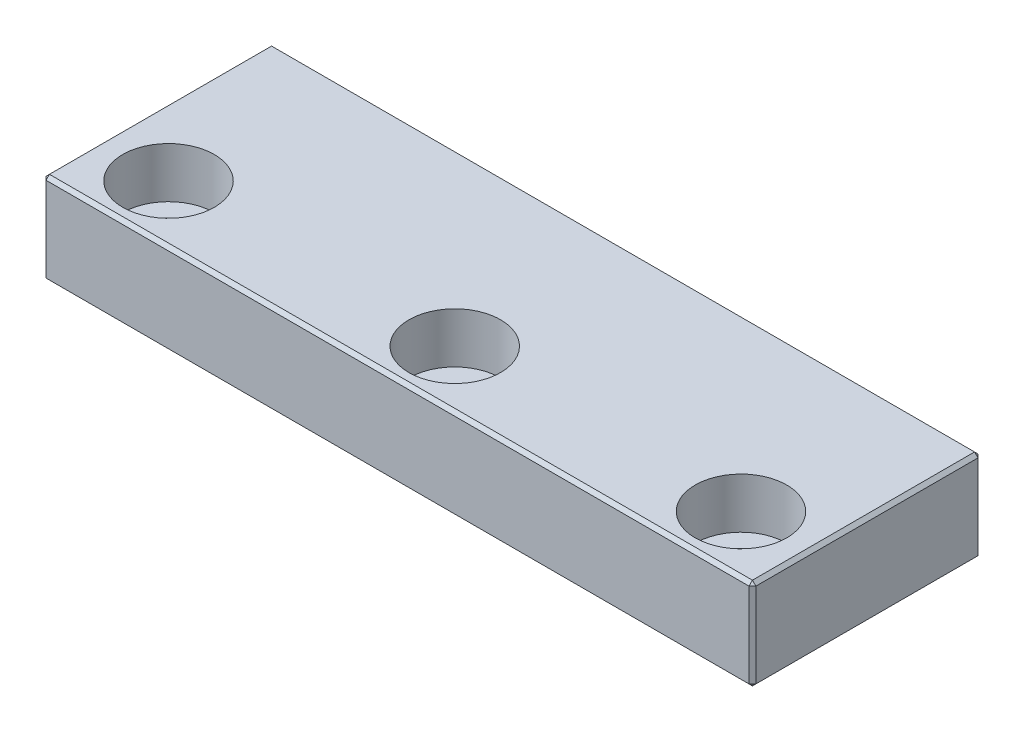
SolidWorks part; units mm, degrees
material "Al6061"
ref_plane "Front" through (0, 0, 0) normal (0, 0, 1) x (1, 0, 0)
ref_plane "Top" through (0, 0, 0) normal (0, 1, 0) x (1, 0, 0)
ref_plane "Right" through (0, 0, 0) normal (1, 0, 0) x (0, 0, -1)
sketch "草图1" plane through (0, 0, 0) normal (0, 1, 0) x (1, 0, 0)
  line L1 (-31, 10) -> (31, 10)
  line L2 (-31, 10) -> (-31, -10)
  line L3 (-31, -10) -> (31, -10)
  line L4 (31, 10) -> (31, -10)
  line L5 (-31, 10) -> (31, -10) construction
  line L6 (-31, -10) -> (31, 10) construction
  point P0 (0, 0)
  dimension "D1" = 62
  dimension "D2" = 20
extrude "凸台-拉伸1" add sketch "草图1" along normal blind 8
hole_wizard "M4 六角凹头螺钉的柱形沉头孔1" positions "草图3" profile "草图2" counterbore size "M4" standard "Iso" end condition through all
sketch "草图3" plane through (0, 8, 0) normal (0, 1, 0) x (1, 0, 0)
  line L0 (0, 0) -> (0, -5) construction
  line L2 (-31, -10) -> (31, -10) construction
  point P0 (-25, -5)
  point P2 (0, -5)
  point P4 (25, -5)
  dimension "D1" = 25
  dimension "D2" = 25
  dimension "D3" = 5
sketch "草图2" plane through (-25, 8, 5) normal (1, 0, 0) x (0, 0, 1)
  line L0 (0, 0) -> (0, 8)
  line L1 (0, 8) -> (2.25, 8)
  line L3 (2.25, 8) -> (2.25, 4.4)
  line L4 (2.25, 4.4) -> (4, 4.4)
  line L5 (4, 4.4) -> (4, 0)
  line L7 (4, 0) -> (0, 0)
  line L11 (0, -6.35) -> (0, 107.95) construction
  dimension "通孔孔直径" = 4.5
  dimension "通孔孔深度" = 8
  dimension "柱形沉头孔直径" = 8
  dimension "柱形沉头孔深度" = 4.4
chamfer "倒角1" distance 0.3 angle 45 12 edges at (-31, 8, 0) (-31, 0, 0) (0, 8, -10) (-31, 4, -10) (0, 0, -10) (31, 8, 0) (31, 4, -10) (31, 0, 0) (-31, 4, 10) (0, 8, 10) (31, 4, 10) (0, 0, 10)
